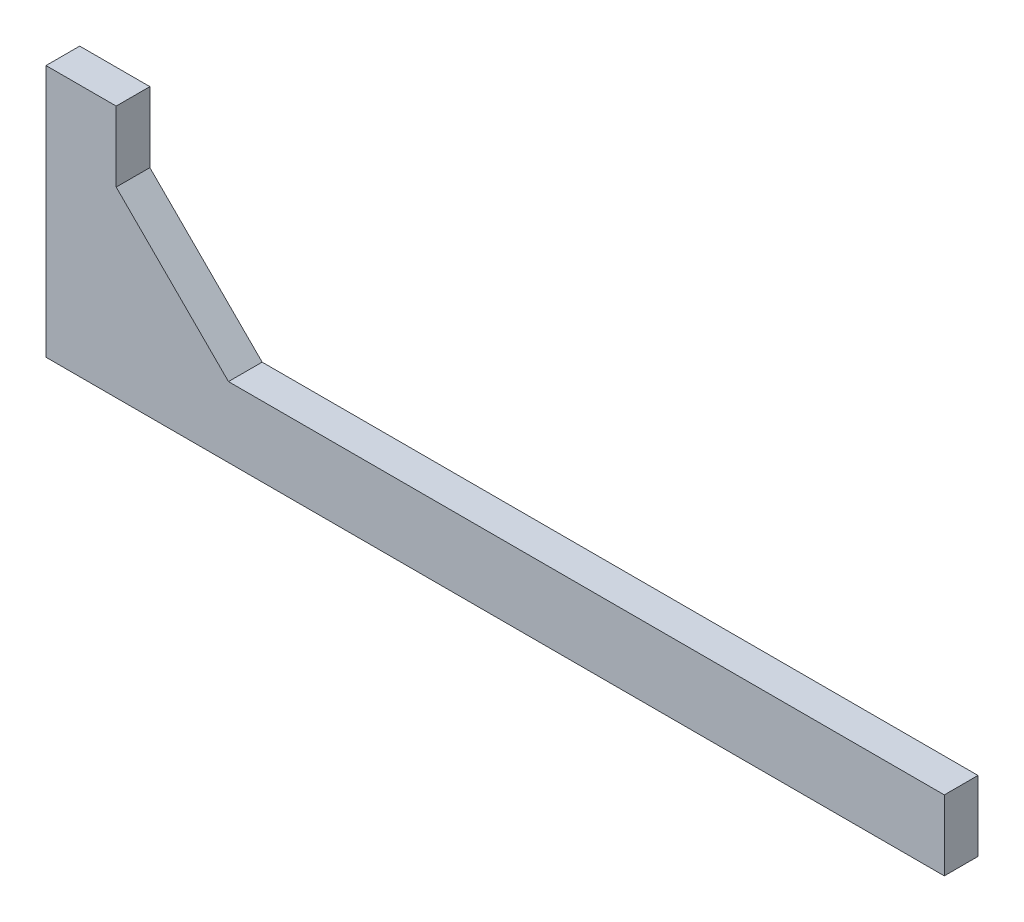
SolidWorks part; units mm, degrees
material "6061 合金"
ref_plane "前视基准面" through (0, 0, 0) normal (0, 0, 1) x (1, 0, 0)
ref_plane "上视基准面" through (0, 0, 0) normal (0, 1, 0) x (1, 0, 0)
ref_plane "右视基准面" through (0, 0, 0) normal (1, 0, 0) x (0, 0, -1)
sketch "草图1" plane through (0, 0, 0) normal (0, 0, 1) x (1, 0, 0)
  line L0 (0, 0) -> (0, 90)
  line L1 (0, 90) -> (25, 90)
  line L2 (25, 90) -> (25, 65)
  line L3 (65, 25) -> (320, 25)
  line L4 (320, 25) -> (320, 0)
  line L5 (320, 0) -> (0, 0)
  line L6 (25, 65) -> (65, 25)
  point P5 (25, 25)
  dimension "D1" = 90
  dimension "D2" = 320
  dimension "D3" = 25
  dimension "D4" = 25
extrude "凸台-拉伸1" add sketch "草图1" along normal mid plane 12
sketch "草图2" plane through (0, 0, 0) normal (-1, 0, 0) x (0, 0, 1)
  line L0 (6, 0) -> (-6, 0) construction
  point P0 (0, 75)
  point P1 (0, 25)
  dimension "D1" = 25
  dimension "D2" = 50
hole_wizard "M8 螺纹孔1" positions "3D草图1" profile "草图5" tap size "M8" standard "GB"
sketch3d "3D草图1"
  point P0 (0, 75, 0)
  point P3 (0, 25, 0)
sketch "草图5" plane through (0, 75, 0) normal (0, 1, 0) x (0, 0, 1)
  line L0 (0, 0) -> (0, 20.7929)
  line L1 (0, 20.7929) -> (3.4, 18.75)
  line L2 (3.4, 18.75) -> (3.4, 0)
  line L5 (3.4, 0) -> (0, 0)
  line L10 (0, 20.7929) -> (-3.4, 18.75) construction
  line L11 (0, -6.35) -> (0, 107.95) construction
  dimension "螺纹孔钻头直径" = 6.8
  dimension "螺纹孔钻头深度" = 18.75
  dimension "导头角度" = 118
cosmetic thread "孔螺蚊线1"
cosmetic thread "孔螺蚊线2"
sketch "草图6" plane through (0, 0, 0) normal (0, -1, 0) x (1, 0, 0)
  line L0 (0, 6) -> (0, -6) construction
  point P0 (45, 0)
  point P1 (165, 0)
  point P2 (285, 0)
  dimension "D1" = 120
  dimension "D2" = 120
  dimension "D3" = 45
hole_wizard "M6 螺纹孔1" positions "3D草图2" profile "草图7" tap size "M6" standard "GB"
sketch3d "3D草图2"
  point P0 (45, 0, 0)
  point P3 (165, 0, 0)
  point P6 (285, 0, 0)
sketch "草图7" plane through (45, 0, 0) normal (1, 0, 0) x (0, 0, -1)
  line L0 (0, 0) -> (0, 16.5022)
  line L1 (0, 16.5022) -> (2.5, 15)
  line L2 (2.5, 15) -> (2.5, 0)
  line L5 (2.5, 0) -> (0, 0)
  line L10 (0, 16.5022) -> (-2.5, 15) construction
  line L11 (0, -6.35) -> (0, 107.95) construction
  dimension "螺纹孔钻头直径" = 5
  dimension "螺纹孔钻头深度" = 15
  dimension "导头角度" = 118
cosmetic thread "孔螺蚊线3"
cosmetic thread "孔螺蚊线4"
cosmetic thread "孔螺蚊线5"
